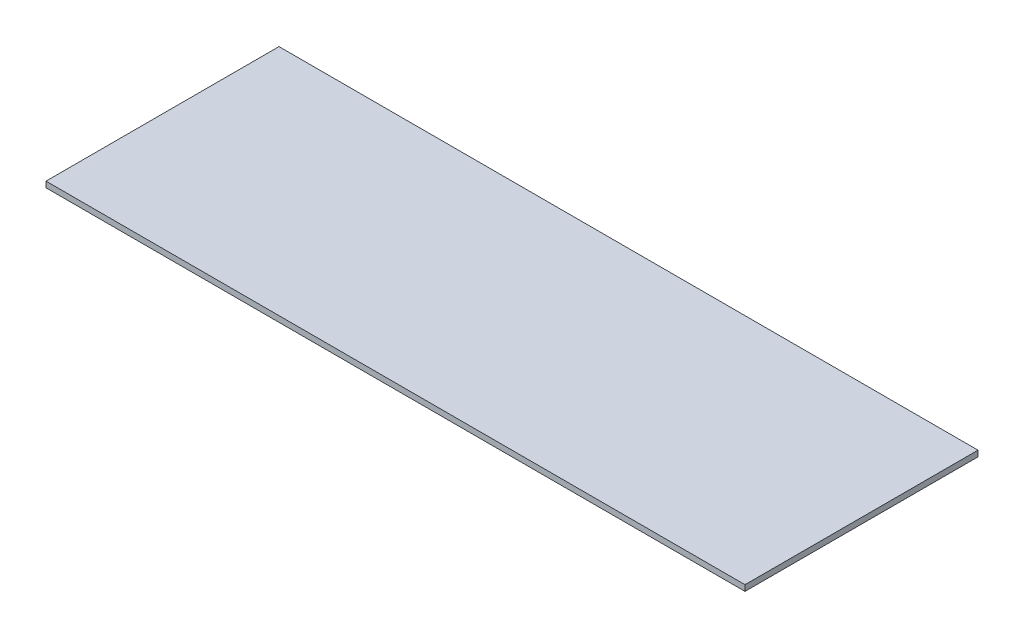
from build123d import *

# Parameters (mm, degrees)
SKETCH1_W           = 1200
SKETCH1_H           = 400
BOSS_EXTRUDE1_DEPTH = 10


with BuildPart() as part:
    # Sketch1 → Boss-Extrude1 (new body)
    with BuildSketch(Plane(origin=(0, 0, 0), x_dir=(1, 0, 0), z_dir=(0, 1, 0))):
        Rectangle(SKETCH1_W, SKETCH1_H)
    extrude(amount=BOSS_EXTRUDE1_DEPTH)


solid = part.part
